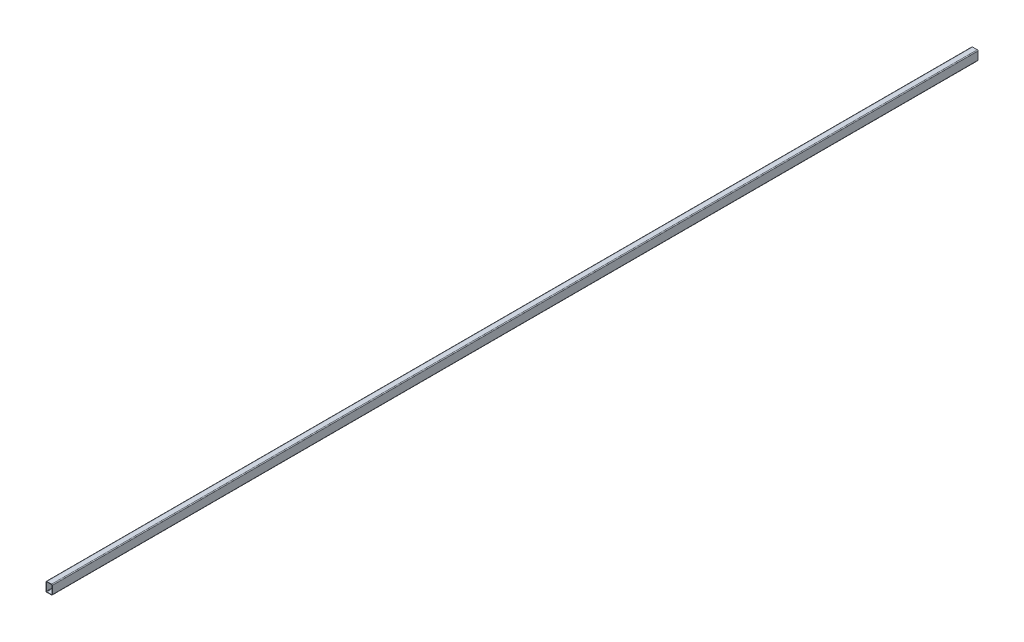
SolidWorks part; units mm, degrees
material "普通碳钢"
ref_plane "Front Plane" through (0, 0, 0) normal (0, 0, 1) x (1, 0, 0)
ref_plane "Top Plane" through (0, 0, 0) normal (0, 1, 0) x (1, 0, 0)
ref_plane "Right Plane" through (0, 0, 0) normal (1, 0, 0) x (0, 0, -1)
sketch "Sketch1" plane through (0, 0, 0) normal (0, 0, 1) x (1, 0, 0)
  line L1 (5, 0) -> (35, 0)
  line L2 (0, 5) -> (0, 55)
  line L3 (5, 60) -> (35, 60)
  line L4 (40, 5) -> (40, 55)
  line L8 (5, 2.5) -> (35, 2.5)
  line L9 (37.5, 5) -> (37.5, 55)
  line L10 (5, 57.5) -> (35, 57.5)
  line L11 (2.5, 5) -> (2.5, 55)
  arc A0 (40, 5) -> (35, 0) centre (35, 5) cw
  arc A1 (0, 55) -> (5, 60) centre (5, 55) cw
  arc A2 (40, 55) -> (35, 60) centre (35, 55) ccw
  arc A3 (5, 0) -> (0, 5) centre (5, 5) cw
  arc A8 (37.5, 5) -> (35, 2.5) centre (35, 5) cw
  arc A9 (37.5, 55) -> (35, 57.5) centre (35, 55) ccw
  arc A10 (2.5, 55) -> (5, 57.5) centre (5, 55) cw
  arc A11 (5, 2.5) -> (2.5, 5) centre (5, 5) cw
  point P7 (40, 0)
  point P10 (0, 60)
  point P13 (40, 60)
  point P16 (0, 0)
  dimension "D3" = 5
  dimension "D4" = 5
  dimension "D5" = 5
  dimension "D6" = 5
  dimension "D1" = 40
  dimension "D2" = 60
  dimension "D7" = 2.5
extrude "Boss-Extrude1" add sketch "Sketch1" along normal blind 5880
